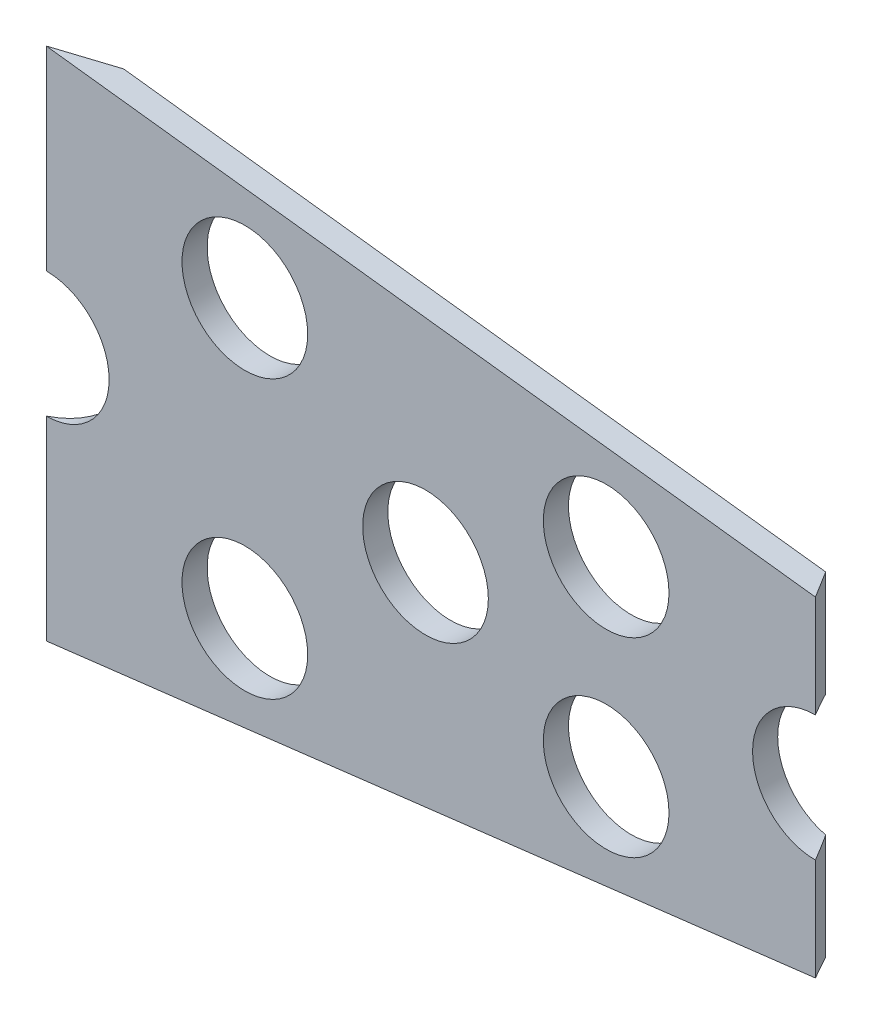
from build123d import *

# Parameters (mm, degrees)
SKETCH1_R           = 40
BOSS_EXTRUDE1_DEPTH = 16
CUT_EXTRUDE2_DEPTH  = 500


with BuildPart() as part:
    # Sketch1 → Boss-Extrude1 (new body)
    with BuildSketch(Plane.XY):
        with BuildLine():
            Line((0, 40), (0, 164))
            Line((0, 164), (489.6, 105))
            Line((489.6, 105), (489.6, 40))
            ThreePointArc((489.6, 40), (449.6, 0), (489.6, -40))
            Line((489.6, -40), (489.6, -105))
            Line((489.6, -105), (0, -164))
            Line((0, -164), (0, -40))
            ThreePointArc((0, -40), (40, 0), (0, 40))
        make_face()
        with Locations((241.4, 0)):
            Circle(SKETCH1_R, mode=Mode.SUBTRACT)
        with Locations((126.4, 88.333889345)):
            Circle(SKETCH1_R, mode=Mode.SUBTRACT)
        with Locations((356.4, 60.617386077)):
            Circle(SKETCH1_R, mode=Mode.SUBTRACT)
        with Locations((126.4, -88.333889345)):
            Circle(SKETCH1_R, mode=Mode.SUBTRACT)
        with Locations((356.4, -60.617386077)):
            Circle(SKETCH1_R, mode=Mode.SUBTRACT)
    extrude(amount=BOSS_EXTRUDE1_DEPTH)

    # Sketch3 → Cut-Extrude2 (cut, along a direction that is not the sketch's normal)
    with BuildSketch(Plane(origin=(19.480184067, -161.652510498, 0), x_dir=(0.9928172236743598, 0.11964096445422229, 0), z_dir=(0.11964096445422229, -0.9928172236743598, 0))):
        Polygon((473.521011443, 16), (464.021011443, 0), (473.521011443, 0), align=None)
        Polygon((-19.62111817, 16), (-19.62111817, 0), (13.87888183, 0), align=None)
    extrude(amount=-CUT_EXTRUDE2_DEPTH, dir=(0, -1, 0), mode=Mode.SUBTRACT)


solid = part.part
